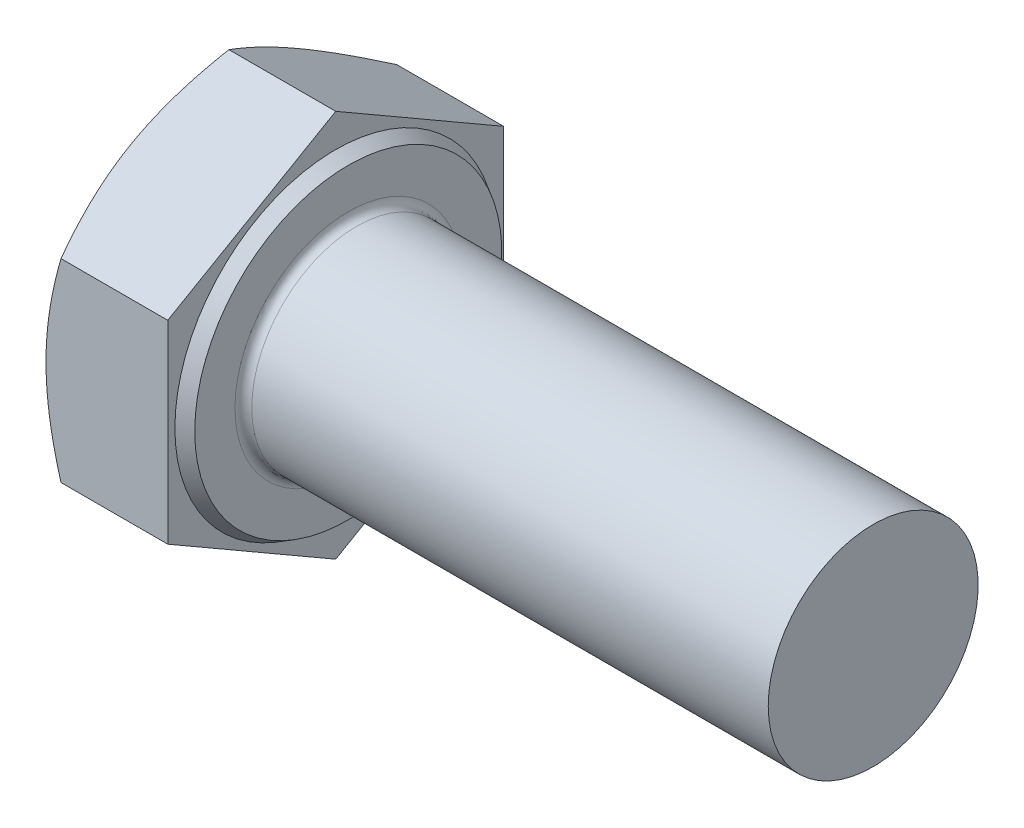
SolidWorks part; units mm, degrees
ref_plane "前视" through (0, 0, 0) normal (0, 0, 1) x (1, 0, 0)
ref_plane "上视" through (0, 0, 0) normal (0, 1, 0) x (1, 0, 0)
ref_plane "右视" through (0, 0, 0) normal (1, 0, 0) x (0, 0, -1)
sketch "草图1" plane through (0, 0, 0) normal (1, 0, 0) x (0, 0, -1)
  line L0 (8, 4.6188) -> (8, -4.6188)
  line L1 (-8, 4.6188) -> (-8, -4.6188)
  line L2 (8, -4.6188) -> (0, -9.2376)
  line L3 (0, -9.2376) -> (-8, -4.6188)
  line L4 (8, 4.6188) -> (0, 9.2376)
  line L5 (0, 9.2376) -> (-8, 4.6188)
  circle A0 centre (0, 0) radius 8.885 construction
  dimension "e" = 17.77
  dimension "s" = 16
  dimension "D2" = 120
  dimension "D3" = 8
  dimension "D4" = 8
  dimension "D5" = 8
extrude "基体-拉伸" add sketch "草图1" along normal blind 6.4
sketch "草图2" plane through (0, 0, 0) normal (0, 0, 1) x (1, 0, 0)
  line L0 (0, 4.6188) -> (0, -4.6188) construction
  line L1 (0, 0) -> (31.4, 0)
  line L2 (0, 0) -> (0, 5)
  line L3 (0, 5) -> (16.4, 5)
  line L4 (31.4, 0) -> (31.4, 3.701)
  line L5 (6.4, 9.2376) -> (6.4, 4.6188) construction
  line L7 (0, 0) -> (41.4, 0) construction
  line L8 (31.4, -3.701) -> (16.4, -5) construction
  line L9 (0, -5) -> (16.4, -5) construction
  line L10 (7.9, 5) -> (7.9, 0) construction
  line L11 (16.4, 15.24) -> (16.4, -1.27) construction
  line L12 (6.4, 4.6188) -> (6.4, -4.6188) construction
  line L13 (16.4, 5) -> (31.4, 5)
  line L14 (31.4, 5) -> (31.4, 3.701)
  dimension "l" = 25
  dimension "d" = 10
  dimension "Minor_dia" = 7.402
  dimension "p" = 1.5
  dimension "b" = 15
  dimension "ds" = 10
revolve "凸台-旋转1" add sketch "草图2" angle 360 about L7
cosmetic thread "螺旋线1" parameters "Thread_length"=26, "Thread_minor"=7.402
sketch "草图3" plane through (0, 0, 0) normal (0, 0, 1) x (1, 0, 0)
  line L0 (0, 8) -> (3.6013, 14.2376)
  line L1 (0, 9.2376) -> (0, 4.6188) construction
  line L2 (3.6013, 14.2376) -> (3.6013, 19.2376)
  line L3 (3.6013, 19.2376) -> (-10, 19.2376)
  line L4 (-10, 19.2376) -> (-10, 8)
  line L5 (-10, 8) -> (0, 8)
  line L6 (0, 0) -> (99.06, 0) construction
  line L7 (6.4, 9.2376) -> (0, 9.2376) construction
  dimension "D1" = 8
  dimension "D2" = 5
  dimension "D3" = 10
  dimension "D4" = 5
  dimension "Head_ch_ang" = 30
revolve "切除-旋转1" cut sketch "草图3" angle 360 about L6
sketch "草图4" plane through (0, 0, 0) normal (0, 0, 1) x (1, 0, 0)
  line L0 (6.4, 0) -> (6.4, 7.315) construction
  line L2 (6.4, -5) -> (6.4, 5) construction
  line L3 (6.4, 9.2376) -> (6.4, 4.6188) construction
  line L4 (6.4, 7.315) -> (5.8, 7.6614)
  line L5 (0, 0) -> (95.25, 0) construction
  line L6 (0, 0) -> (41.4, 0) construction
  line L9 (5.8, 7.6614) -> (5.8, 9.2376)
  line L10 (6.4, 9.2376) -> (0.7145, 9.2376) construction
  line L11 (5.8, 9.2376) -> (6.4, 9.2376)
  line L12 (6.4, 9.2376) -> (6.4, 7.315)
  dimension "D1" = 120
  dimension "c" = 0.6
  dimension "dw" = 14.63
revolve "切除-旋转3" cut sketch "草图4" angle 360 about L5
fillet "圆角" radius 0.4 1 edges at (6.4, 0, -5)
sketch "草图6" plane through (0, 0, 0) normal (0, 0, 1) x (1, 0, 0)
  line L0 (0, 0) -> (31.4, 0) construction
  line L1 (31.4, -5) -> (31.4, 5) construction
  line L2 (31.4, 0) -> (31.4, 5) construction
  line L4 (30.65, 5) -> (32.15, 5)
  line L5 (30.65, 5) -> (31.4, 3.701)
  line L6 (31.4, 3.701) -> (32.15, 5)
  dimension "D1" = 1.5
revolve "切除-旋转4" [suppressed] cut sketch "草图6" angle 360 about L0
pattern_linear "阵列(线性)1" [suppressed]
